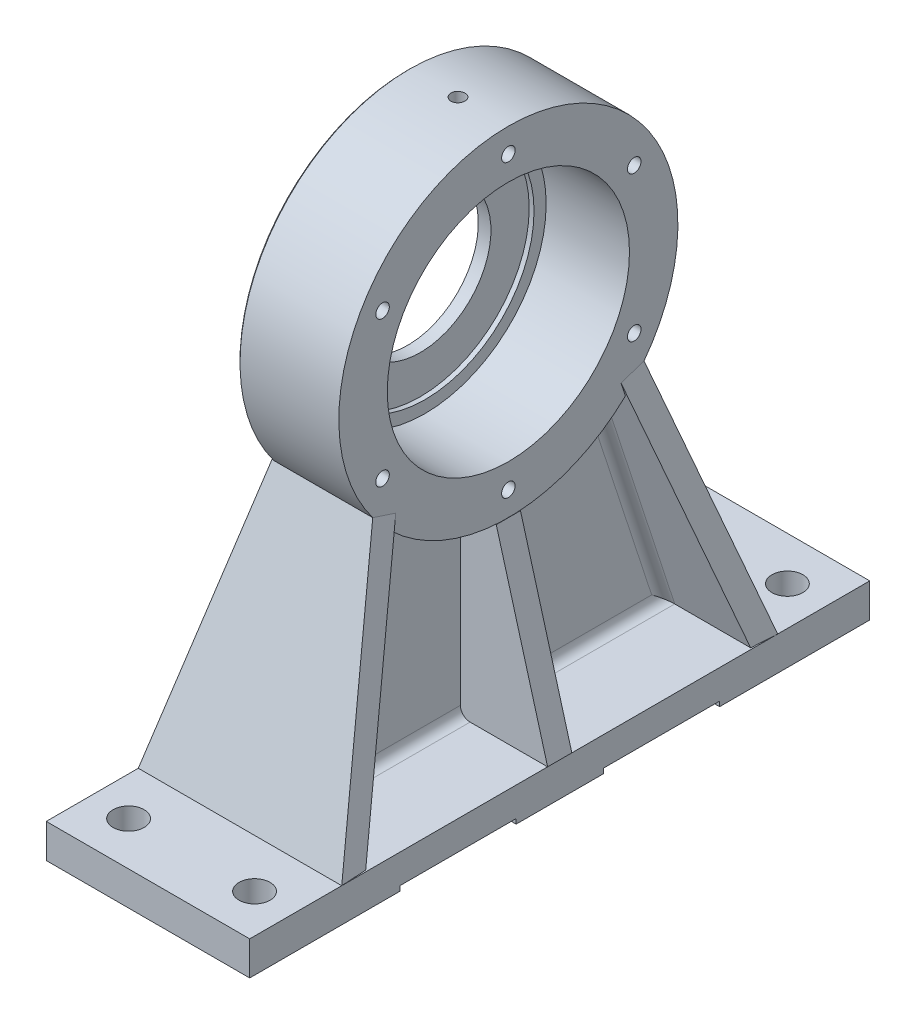
from build123d import *

# Parameters (mm, degrees)
BOSS_EXTRUDE1_DEPTH         = 105
BOSS_EXTRUDE2_DEPTH         = 15
BOSS_EXTRUDE6_DEPTH         = 12.5
BOSS_EXTRUDE3_DEPTH         = 25
FILLET1_R                   = 10
SKETCH7_R                   = 16
CUT_EXTRUDE1_DEPTH          = 637.41574462
M16_TAPPED_HOLE1_AT_2_COUNT = 2
M16_TAPPED_HOLE1_AT_2_PITCH = 150
M16_TAPPED_HOLE1_AT_3_COUNT = 2
M16_TAPPED_HOLE1_AT_3_PITCH = 259.807621135
M16_TAPPED_HOLE1_AT_4_COUNT = 2
M16_TAPPED_HOLE1_AT_4_PITCH = 300
M16_TAPPED_HOLE1_AT_5_COUNT = 2
M16_TAPPED_HOLE1_AT_5_PITCH = 259.807621135
M16_TAPPED_HOLE1_AT_6_COUNT = 2
M16_TAPPED_HOLE1_AT_6_PITCH = 150
CHAMFER1_SIZE               = 2


with BuildPart() as part:
    # Sketch1 → Revolve1 (revolve)
    with BuildSketch(Plane.XY, mode=Mode.PRIVATE) as revolve1_sk:
        Polygon((-52, 73), (-52, 175), (52, 175), (52, 125), (-34, 125), (-34, 112.5), (-39, 112.5), (-39, 73), align=None)
    revolve(revolve1_sk.sketch.rotate(Axis((0, 0, 0), (1, 0, 0)), 90), axis=Axis((0, 0, 0), (1, 0, 0)))



with BuildPart() as body_2:
    # Sketch2 → Boss-Extrude1 (new, symmetric)
    with BuildSketch(Plane(origin=(0, 0, 0), x_dir=(0, 0, -1), z_dir=(1, 0, 0))):
        Polygon((-320, -400), (-320, -365), (320, -365), (320, -400), (165, -400), (165, -395), (45, -395), (45, -400), (-45, -400), (-45, -395), (-165, -395), (-165, -400), align=None)
    extrude(amount=BOSS_EXTRUDE1_DEPTH, both=True)


with BuildPart() as part_1:
    add(part.part)

    add(body_2.part)  # Boss-Extrude2 merges body 2
    # Sketch3 → Boss-Extrude2 (add, symmetric)
    with BuildSketch(Plane(origin=(0, 0, 0), x_dir=(0, 0, -1), z_dir=(1, 0, 0))):
        with BuildLine():
            Line((-140, -105), (-225, -365))
            Line((-225, -365), (225, -365))
            Line((225, -365), (140, -105))
            ThreePointArc((140, -105), (0, -175), (-140, -105))
        make_face()
    extrude(amount=BOSS_EXTRUDE2_DEPTH, both=True)

    # Sketch4 → Boss-Extrude3 (add)
    with BuildSketch(Plane(origin=(0, 31.211159372, 95.469428667), x_dir=(1, 0, 0), z_dir=(0, 0.3107388563074221, 0.9504953251756451))):
        Polygon((-52, -143.305449026), (52, -143.305449026), (105, -416.847036358), (-105, -416.847036358), align=None)
    boss_extrude3 = extrude(amount=-BOSS_EXTRUDE3_DEPTH)

    # Mirror1: Boss-Extrude3 across plane
    add(boss_extrude3.mirror(Plane.XY))

    # Fillet1
    fillet1_edges = [part_1.edges().sort_by_distance(p)[0] for p in [
        (15, -365, 0),
        (-15, -365, 0),
        (15, -245.821962461, 159.735873561),
        (-15, -175, 0),
        (15, -175, 0),
        (-15, -245.821962461, -159.735873561),
        (15, -245.821962461, -159.735873561),
    ]]
    fillet(fillet1_edges, radius=FILLET1_R)

    # Sketch7 → Cut-Extrude1 (cut, through all)
    with BuildSketch(Plane(origin=(0, -365, 0), x_dir=(1, 0, 0), z_dir=(0, 1, 0))):
        with Locations(Location((-65, 275, 0), (0, 0, 270))):
            Circle(SKETCH7_R)
        with Locations(Location((65, 275, 0), (0, 0, 270))):
            Circle(SKETCH7_R)
        with Locations(Location((-65, -275, 0), (0, 0, 270))):
            Circle(SKETCH7_R)
        with Locations(Location((65, -275, 0), (0, 0, 270))):
            Circle(SKETCH7_R)
    extrude(amount=-CUT_EXTRUDE1_DEPTH, mode=Mode.SUBTRACT)

    # Sketch9 → M16 Tapped Hole1 (revolve, cut)
    with BuildSketch(Plane(origin=(52, -75, 129.903810568), x_dir=(0, 0, -1), z_dir=(0, 1, 0))):
        Polygon((0, 0), (0, 42.206024333), (7, 38), (7, 0), align=None)
    m16_tapped_hole1 = revolve(axis=Axis((58.35, -75, 129.903810568), (-1, 0, 0)), mode=Mode.SUBTRACT)

    # M16 Tapped Hole1 at 2: M16 Tapped Hole1 ×2
    with Locations(*[Vector(0, -0.5000000000000074, -0.8660254037844345) * (i * M16_TAPPED_HOLE1_AT_2_PITCH) for i in range(1, M16_TAPPED_HOLE1_AT_2_COUNT)]):
        add(m16_tapped_hole1, mode=Mode.SUBTRACT)

    # M16 Tapped Hole1 at 3: M16 Tapped Hole1 ×2
    with Locations(*[(0, 0, -i * M16_TAPPED_HOLE1_AT_3_PITCH) for i in range(1, M16_TAPPED_HOLE1_AT_3_COUNT)]):
        add(m16_tapped_hole1, mode=Mode.SUBTRACT)

    # M16 Tapped Hole1 at 4: M16 Tapped Hole1 ×2
    with Locations(*[Vector(0, 0.499999999999996, -0.8660254037844409) * (i * M16_TAPPED_HOLE1_AT_4_PITCH) for i in range(1, M16_TAPPED_HOLE1_AT_4_COUNT)]):
        add(m16_tapped_hole1, mode=Mode.SUBTRACT)

    # M16 Tapped Hole1 at 5: M16 Tapped Hole1 ×2
    with Locations(*[Vector(0, 0.8660254037844365, -0.5000000000000039) * (i * M16_TAPPED_HOLE1_AT_5_PITCH) for i in range(1, M16_TAPPED_HOLE1_AT_5_COUNT)]):
        add(m16_tapped_hole1, mode=Mode.SUBTRACT)

    # M16 Tapped Hole1 at 6: M16 Tapped Hole1 ×2
    with Locations(*[(0, i * M16_TAPPED_HOLE1_AT_6_PITCH, 0) for i in range(1, M16_TAPPED_HOLE1_AT_6_COUNT)]):
        add(m16_tapped_hole1, mode=Mode.SUBTRACT)

    # Sketch12 → M16x1.5 Tapped Hole1 (revolve, cut)
    with BuildSketch(Plane(origin=(0, 175, 0), x_dir=(0, 0, 1), z_dir=(1, 0, 0))):
        Polygon((0, 0), (0, 60.856239488), (7.25, 56.5), (7.25, 0), align=None)
    revolve(axis=Axis((0, 181.35, 0), (0, -1, 0)), mode=Mode.SUBTRACT)

    # Chamfer1
    chamfer1_edges = [part_1.edges().sort_by_distance(p)[0] for p in [
        (-52, 175, 0),
    ]]
    chamfer(chamfer1_edges, length=CHAMFER1_SIZE)


with BuildPart() as body_2_2:
    # Sketch6 → Boss-Extrude6 (new, symmetric)
    with BuildSketch(Plane.XY):
        Polygon((105, -365), (52, -175), (-52, -175), (-105, -365), align=None)
    extrude(amount=BOSS_EXTRUDE6_DEPTH, both=True)


solid = Compound([part_1.part, body_2_2.part])
